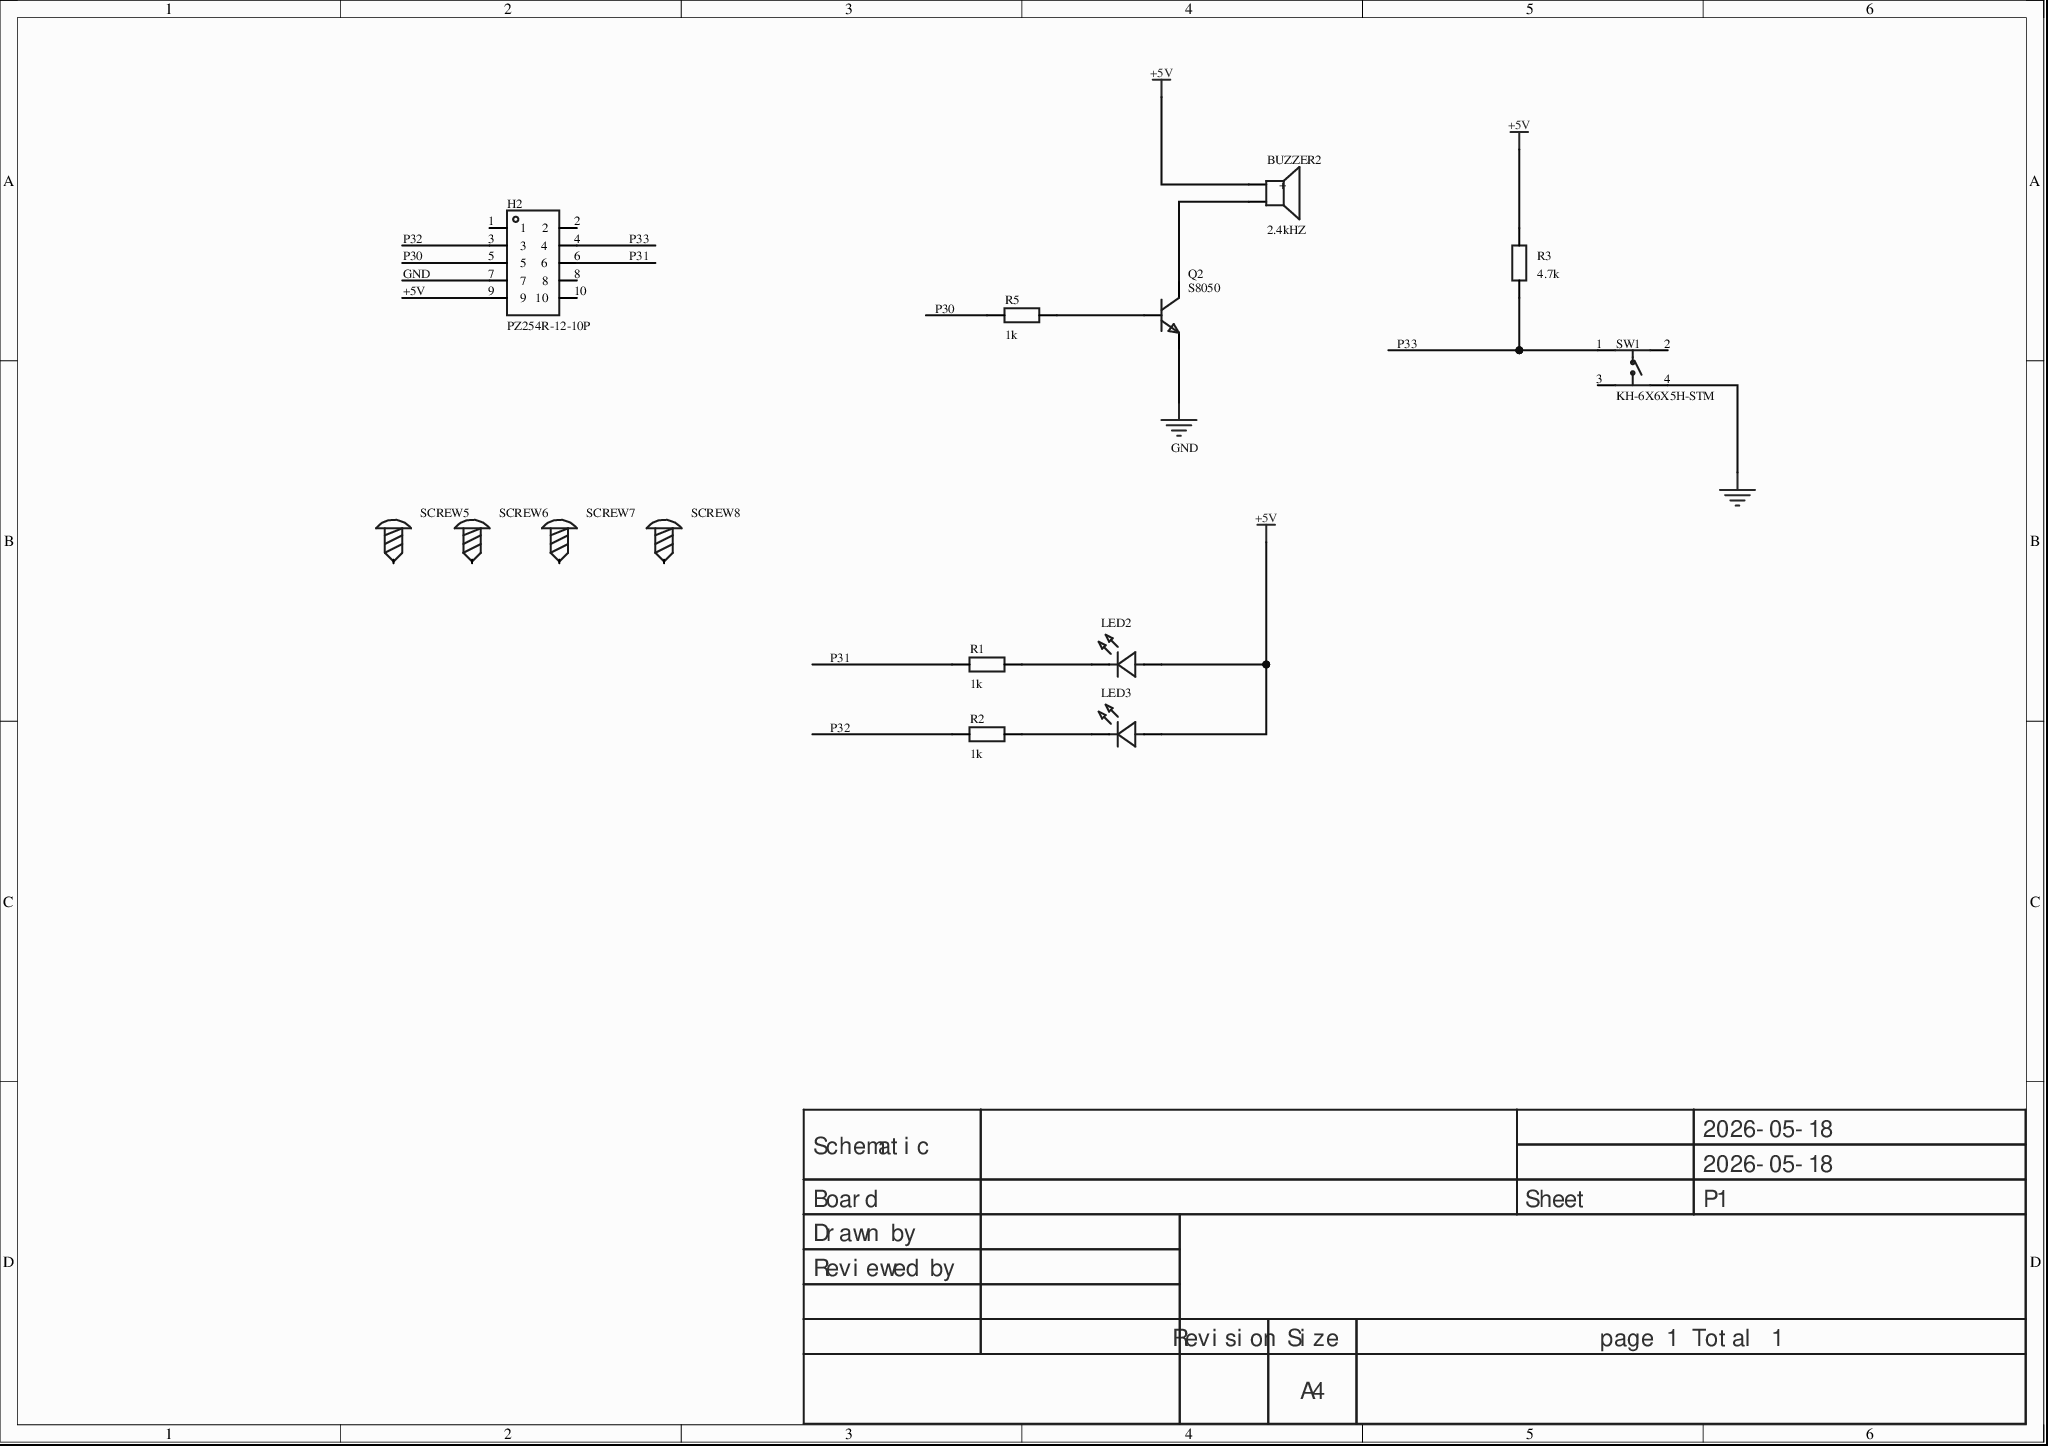
[diagram p0: MISC89027-3.schdoc]
# Altium project MISC89027-2.PrjPcb
1 sheet, 14 parts. Net scope: global (net labels, ports and power ports of the same name join across sheets).
Board file: MISC89027.pcbdoc

## Sheet MISC89027-3.schdoc
size 297 x 209 mm; Version: V1.0; @Project Name: MISC89027; @Page Count: 1; @Update Date: 2026-05-18; @Create Date: 2026-05-18; @Schematic Name: MISC89027; @Page No: 1; @Create Time: 10:46:10; @Update Time: 10:46:10; @Board Name: MISC89027

### Parts
BUZZER2  2.4kHZ  [BUZ-TH_BD12.0-P7.60-D0.6-FD]
H2  PZ254R-12-10P  [HDR-TH_10P-P2.54-H-M-R2-C5-S2.54]
LED2  GL0805UR01  [LED0805-R-RD_RED]  (value not drawn)
LED3  GL0805UR01  [LED0805-R-RD_RED]  (value not drawn)
Q2  S8050  [SOT-23-3_L2.9-W1.3-P1.90-LS2.3-BR]
R1  1k  [R0805]
R2  1k  [R0805]
R3  4.7k  [R0805]
R5  1k  [R0805]
SCREW5  (no value)  [M3螺丝]
SCREW6  (no value)  [M3螺丝]
SCREW7  (no value)  [M3螺丝]
SCREW8  (no value)  [M3螺丝]
SW1  KH-6X6X5H-STM  [SW-SMD_4P-L6.0-W6.0-P4.50-LS9.0_H5.0]

### Nets
+5V: BUZZER2.1(+) LED2.1(A) LED3.1(A) R3.2
GND: Q2.2(E) SW1.4
NetBUZZER2_2: BUZZER2.2 Q2.3(C)
NetLED2_2: LED2.2(C) R1.2
NetLED3_2: LED3.2(C) R2.2
NetQ2_1: Q2.1(B) R5.2
NetR3_1: R3.1 SW1.1

Not connected (* = marked no-connect by the designer): H2 1* 2* 3 4 5 6 7 8* 9 10*; R1 1; R2 1; R5 1; SCREW5 1; SCREW6 1; SCREW7 1; SCREW8 1; SW1 2* 3*

### Notes on the sheet
- P32
- P30
- P33
- P31
- GND
- +5V
- (near R5) P30
- 2026-05-18
- Schematic
- Board
- Sheet
- P1
- Drawn by
- Reviewed by
- Revision
- Size
- A4
- page 1 Total 1

### Library data of the parts
BUZZER2 = TMB12A05_C96093: Drive mode: active (built-in driver circuit); construction: electromagnetic; rated voltage: 5V; operating voltage: 4V~8V; frequency: 2300Hz; sound pressure (SPL): 85dB@5V,10cm; diameter (φD): 12mm; height: 9.8mm;; Manufacturer: 华能; 3D Model: 16ab50e14c5b4f2c986c135bdba60e370819f05c4eef4c71ace90d822a990e87; 3D Model Transform: 472.4,472.2,0,90,0,0,-0.8,0,-177.2; AddInBom: yes; ModelName: BUZ-TH_D12.0-H9.5-P7.60; Symbol: TMB12A05; Device: TMB12A05_C96093; LCSC Part Name: TMB12A05; Supplier Part: C96093; Manufacturer Part: TMB12A05; Supplier Footprint: 插件,P=7.6mm; JLCPCB Part Class: Extended Part; Datasheet: https://atta.szlcsc.com/upload/public/pdf/source/20170522/1495448324811.pdf; Supplier: LCSC; Oscillator Circuit: Active (built-in driver circuit); Technology Type: Electromagnetic; Rated Voltage: 5V; Operating Voltage: 4V~8V; Value: 2300Hz; Sound Pressure Level (SPL): 85dB@5V,10cm; Diameter (φD): 12mm; Height: 9.8mm; ConvertToPcb: yes; FootprintName: BUZ-TH_BD12.0-P7.60-D0.6-FD
H2 = PZ254R-12-10P: Pin structure: 2x5P; pitch: 2.54mm; row spacing: 2.54mm; round/square pin: square pin; mounting: right-angle; rows: dual row; total pins: 10P; rated current: -; rated voltage: -; mating pin length: 6mm; insulation height: 2.5mm; contact material: brass; contact plating: -; operating temperature: -40℃~+105℃; color: black;; Manufacturer: XFCN(兴飞); AddInBom: yes; ModelId: 66dcb0d10d864a6fa7f7fb003119df450819f05c4eef4c71ace90d822a990e87; ModelName: HDR-TH_10P-P2.54-M-WI-2X5P; ModelTransform: 499.999,507.873,0,0,0,0,0,-188.976,-118.11; Symbol: PZ254R-12-10P; Device: PZ254R-12-10P; LCSC Part Name: 2x5P 间距:2.54mm 方针 弯插; SupplierPart: C492433; ManufacturerPart: PZ254R-12-10P; Supplier Footprint: 弯插,P=2.54mm; JLCPCB Part Class: Extended Part; Datasheet: https://item.szlcsc.com/datasheet/PZ254R-12-10P/502989.html; Supplier: LCSC; ConvertToPcb: yes; FootprintName: HDR-TH_10P-P2.54-H-M-R2-C5-S2.54; Pin Structure: 2x5P; Pitch: 2.54mm; Row Spacing: 2.54mm; Circluar Pins/Square Pins: Square pin; Mounting Type: Right-angle; Number of Rows: Dual row; Number of Pins: 10P; Current Rating: -; Voltage Rating (Max): -; Length of Mating Pin: 6mm; Insulation Height: 2.5mm; Contact Material: Brass; Contact Plating: -; Operating Temperature: -40℃~+105℃; Color: Black
LED2 LED3 = GL0805UR01: Lamp holder type: 2mmx1.25mm square lamp holder; illumination color: red; forward voltage (Vf): 2.1V; power: -; forward current: 20mA; wavelength: 618nm~624nm; diode configuration: independent diode; lens color: clear lens; color temperature: -; luminous intensity: 100mcd; viewing angle: 120°; mounting: surface mount; operating temperature: -40℃~+85℃;; Manufacturer: Guiguang light(桂光光电); AddInBom: yes; ModelId: f010e90d36544999ab4e363fdba5b4900819f05c4eef4c71ace90d822a990e87; ModelTransform: 78.74,49.21644,0,0,0,0,0,0,0; Symbol: GL0805UR01; Device: GL0805UR01; LCSC Part Name: 0805 红灯 高亮; SupplierPart: C51933307; ManufacturerPart: GL0805UR01; Supplier Footprint: 0805; JLCPCB Part Class: Extended Part; Datasheet: https://item.szlcsc.com/datasheet/GL0805UR01/54646003.html; Supplier: LCSC; ConvertToPcb: yes; FootprintName: LED0805-R-RD_RED; ModelName: LED0805-R-RD_RED; Lamp Holder Type: 2mmx1.25mm square lamp holder; Illumination Color: Red; Voltage - Forward(Vf): 2.1V; Power(Watts): -; Forward Current: 20mA; Wavelength - Dominant: 618nm~624nm; Peak Wavelength: -; Diode Configuration: Independent diode; Lens Color: Clear lens; Color Temperature: -; Luminous Intensity: 100mcd; Viewing Angle: 120°; Mounting Style: Surface mount; Operating Temperature: -40℃~+85℃
Q2 = S8050_C20069125: Transistor type: NPN; collector current (Ic): 500mA; collector-emitter breakdown voltage (Vceo): 25V; power dissipation (Pd): 300mW; DC current gain (hFE): 120@50mA,1.0V;; Manufacturer: R+O(宏嘉诚); AddInBom: yes; ModelId: 5504beb8757f4de79731898ec55d3e540819f05c4eef4c71ace90d822a990e87; ModelTransform: 114.173,90.551,0,90,0,0,0,0,0; Transition frequency(fT): 100MHz; Current - Collector Cutoff: 100nA; Vce Saturation(VCE(sat)): 600mV@500mA,50mA; Emitter-Base Voltage(Vebo): 5V; Symbol: S8050_C20069125; Device: S8050_C20069125; LCSC Part Name: hFE:200-350，丝印:J3Y NPN 500mA 25V; SupplierPart: C20069125; ManufacturerPart: S8050; Supplier Footprint: SOT-23; JLCPCB Part Class: Extended Part; Datasheet: https://item.szlcsc.com/datasheet/S8050/21397163.html; Supplier: LCSC; ConvertToPcb: yes; FootprintName: SOT-23-3_L2.9-W1.3-P1.90-LS2.3-BR; ModelName: SOT-23-3_L2.9-W1.3-P1.90-LS2.3-BR; type: NPN; Current - Collector(Ic): 500mA; Collector - Emitter Voltage VCEO: 25V; Pd - Power Dissipation: 300mW; DC Current Gain: 120@50mA,1.0V; Operating Temperature: -55℃~+150℃
R1 R2 R5 = Res_0805: Symbol: Resistor; Value: 10K; 3D Model: 37a81e68749a4138bd2dfa6897b24b850819f05c4eef4c71ace90d822a990e87; 3D Model Transform: 78.74,51.181,0,0,0,0,0,-0.0005,0; ConvertToPcb: yes; ModelName: R0805_L2.0-W1.3-H0.6; Device: Res_0805; Supplier Footprint: 0805; AddInBom: yes; FootprintName: R0805
R3 = Res_0805: Symbol: Resistor; ConvertToPcb: yes; Value: 10K; ModelId: 37a81e68749a4138bd2dfa6897b24b850819f05c4eef4c71ace90d822a990e87; ModelName: R0805_L2.0-W1.3-H0.6; ModelTransform: 78.74,51.181,0,0,0,0,0,-0.0005,0; Device: Res_0805; AddInBom: yes; Supplier Footprint: 0805; FootprintName: R0805
SCREW5-SCREW8 = M3螺丝: Symbol: Screw hole; Device: M3 screw; ConvertToPcb: yes; Supplier Footprint: 插件; AddInBom: yes; FootprintName: M3 screw
SW1 = KH-6X6X5H-STM: Circuit: SPDT; Button shape: round; Mounting: upright SMD; Length: 6mm; Width: 6mm; Height: 5mm; Bracket: none; Contact current: 50mA; Rated voltage: 12V; Life: 8万 cycles;; Manufacturer: kinghelm(金航标); AddInBom: yes; ModelId: 46371efb35684031937580a0045530ec0819f05c4eef4c71ace90d822a990e87; ModelTransform: 354.33,236.25937,0,0,0,0,0,0,0; Actuator Style: Round button; with Bracket: No bracket; Actuator/Cap Color: Black; Symbol: KH-6X6X5H-STM; Device: KH-6X6X5H-STM; LCSC Part Name: 6*6*5mm 立贴 轻触开关; SupplierPart: C2837531; ManufacturerPart: KH-6X6X5H-STM; Supplier Footprint: SMD-4P,6x6mm; JLCPCB Part Class: Extended Part; Datasheet: https://item.szlcsc.com/datasheet/KH-6X6X5H-STM/3009601.html; Supplier: LCSC; ConvertToPcb: yes; FootprintName: SW-SMD_4P-L6.0-W6.0-P4.50-LS9.0_H5.0; ModelName: SW-SMD_4P-L6.0-W6.0-P4.50-LS9.0_H5.0; Mounting Type: Upright SMD; Switch Height: 5mm; Contact Current: 50mA; Voltage Rating: 12V; Termination Style: Gull-wing; Life: 8万 cycles